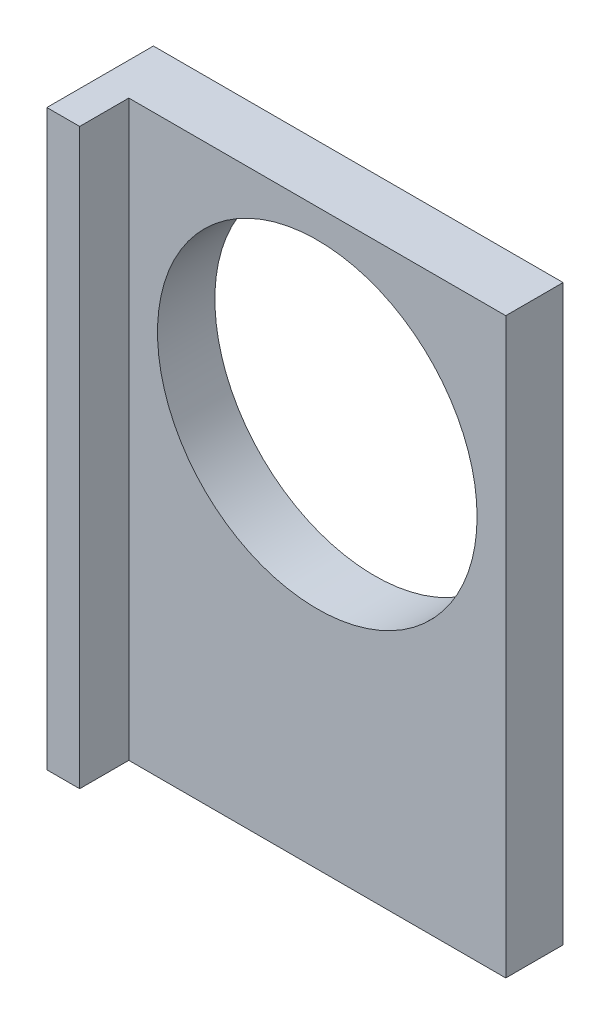
SolidWorks part; units mm, degrees
ref_plane "前视基准面" through (0, 0, 0) normal (0, 0, 1) x (1, 0, 0)
ref_plane "上视基准面" through (0, 0, 0) normal (0, 1, 0) x (1, 0, 0)
ref_plane "右视基准面" through (0, 0, 0) normal (1, 0, 0) x (0, 0, -1)
sketch "草图1" plane through (0, 0, 0) normal (0, 0, 1) x (1, 0, 0)
  line L1 (-50, -70) -> (50, -70)
  line L2 (-50, -70) -> (-50, 70)
  line L3 (-50, 70) -> (50, 70)
  line L4 (50, -70) -> (50, 70)
  line L5 (-50, -70) -> (50, 70) construction
  line L6 (-50, 70) -> (50, -70) construction
  point P0 (0, 0)
  dimension "D1" = 100
  dimension "D2" = 140
extrude "凸台-拉伸1" add sketch "草图1" along normal blind 14
sketch "草图2" plane through (0, 0, 14) normal (0, 0, 1) x (1, 0, 0)
  line L0 (50, 70) -> (-50, 70) construction
  line L1 (50, -70) -> (50, 70) construction
  circle A0 centre (4, 24) radius 39
  dimension "D1" = 78
  dimension "D2" = 46
  dimension "D3" = 46
extrude "切除-拉伸1" cut sketch "草图2" against normal up to next
sketch "草图3" plane through (0, 0, 14) normal (0, 0, 1) x (1, 0, 0)
  line L0 (-50, -70) -> (50, -70) construction
  line L1 (-50, 70) -> (-42, 70)
  line L2 (-50, 70) -> (-50, -70)
  line L3 (-50, -70) -> (-42, -70)
  line L4 (-42, 70) -> (-42, -70)
  dimension "D1" = 8
extrude "凸台-拉伸2" add sketch "草图3" along normal blind 12
